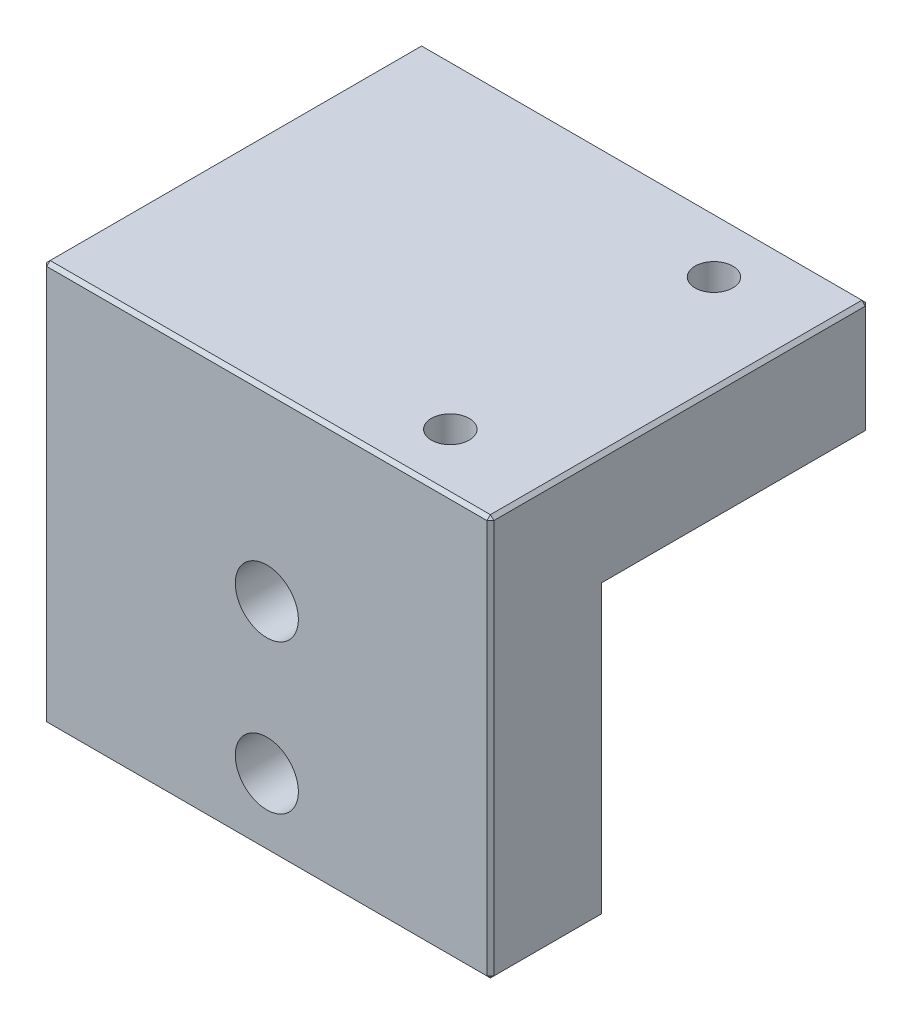
SolidWorks part; units mm, degrees
material "Al6061"
ref_plane "Front" through (0, 0, 0) normal (0, 0, 1) x (1, 0, 0)
ref_plane "Top" through (0, 0, 0) normal (0, 1, 0) x (1, 0, 0)
ref_plane "Right" through (0, 0, 0) normal (1, 0, 0) x (0, 0, -1)
sketch "草图1" plane through (0, 0, 0) normal (0, 1, 0) x (1, 0, 0)
  line L1 (-19.5, 16.5) -> (19.5, 16.5)
  line L2 (-19.5, 16.5) -> (-19.5, -16.5)
  line L3 (-19.5, -16.5) -> (19.5, -16.5)
  line L4 (19.5, 16.5) -> (19.5, -16.5)
  line L5 (-19.5, 16.5) -> (19.5, -16.5) construction
  line L6 (-19.5, -16.5) -> (19.5, 16.5) construction
  point P0 (0, 0)
  dimension "D1" = 39
  dimension "D2" = 33
extrude "凸台-拉伸1" add sketch "草图1" along normal blind 10
sketch "草图2" plane through (0, 0, 0) normal (0, -1, 0) x (1, 0, 0)
  line L0 (19.5, 16.5) -> (19.5, -16.5) construction
  line L1 (-19.5, 16.5) -> (19.5, 16.5)
  line L2 (-19.5, 16.5) -> (-19.5, 6.5)
  line L3 (-19.5, 6.5) -> (19.5, 6.5)
  line L4 (19.5, 16.5) -> (19.5, 6.5)
  dimension "D1" = 10
extrude "凸台-拉伸2" add sketch "草图2" along normal blind 25
hole_wizard "M4 螺纹孔1" positions "草图4" profile "草图3" tap size "M4" standard "Iso"
sketch "草图4" plane through (0, 10, 0) normal (0, 1, 0) x (1, 0, 0)
  line L0 (19.5, -16.5) -> (19.5, 16.5) construction
  line L1 (0, 0) -> (19.5, 0) construction
  point P0 (11, 11.5)
  point P2 (11, -11.5)
  dimension "D1" = 8.5
  dimension "D2" = 23
sketch "草图3" plane through (11, 10, -11.5) normal (1, 0, 0) x (0, 0, 1)
  line L0 (0, 0) -> (0, 14.4914)
  line L1 (0, 14.4914) -> (1.65, 13.5)
  line L2 (1.65, 13.5) -> (1.65, 0)
  line L5 (1.65, 0) -> (0, 0)
  line L10 (0, 14.4914) -> (-1.65, 13.5) construction
  line L11 (0, -6.35) -> (0, 107.95) construction
  dimension "螺纹孔钻头直径" = 3.3
  dimension "螺纹孔钻头深度" = 13.5
  dimension "导头角度" = 118
cosmetic thread "孔螺蚊线1" parameters "D1"=10, "D2"=4
cosmetic thread "孔螺蚊线2" parameters "D1"=10, "D2"=4
hole_wizard "M5 六角凹头螺钉的柱形沉头孔1" positions "草图6" profile "草图5" counterbore size "M5" standard "Iso" end condition through all
sketch "草图6" plane through (0, 0, 6.5) normal (0, 0, -1) x (-1, 0, 0)
  line L0 (0, 0) -> (0, -6) construction
  line L2 (19.5, -25) -> (-19.5, -25) construction
  point P0 (0, -6)
  point P2 (0, -19)
  dimension "D1" = 13
  dimension "D2" = 6
sketch "草图5" plane through (0, -6, 6.5) normal (1, 0, 0) x (0, 1, 0)
  line L0 (0, 0) -> (0, 10)
  line L1 (0, 10) -> (2.75, 10)
  line L3 (2.75, 10) -> (2.75, 5.4)
  line L4 (2.75, 5.4) -> (5, 5.4)
  line L5 (5, 5.4) -> (5, 0)
  line L7 (5, 0) -> (0, 0)
  line L11 (0, -6.35) -> (0, 107.95) construction
  dimension "通孔孔直径" = 5.5
  dimension "通孔孔深度" = 10
  dimension "柱形沉头孔直径" = 10
  dimension "柱形沉头孔深度" = 5.4
chamfer "倒角1" distance 0.3 angle 45 17 edges at (0, -25, 16.5) (0, -25, 6.5) (0, 10, -16.5) (0, 0, -16.5) (-19.5, 5, -16.5) (-19.5, 10, 0) (-19.5, -25, 11.5) (-19.5, -7.5, 16.5) (19.5, 10, 0) (19.5, 5, -16.5) (19.5, -25, 11.5) (19.5, -7.5, 16.5) (0, 10, 16.5)
